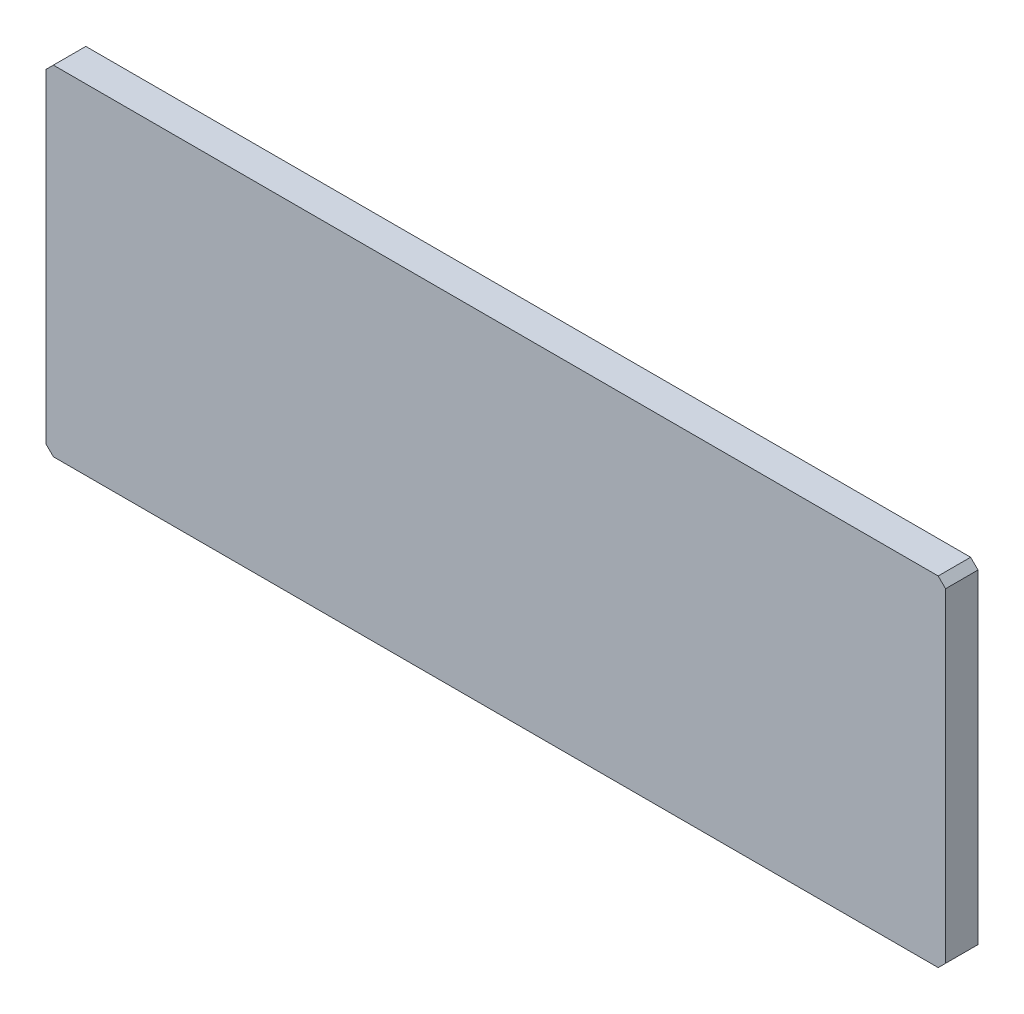
SolidWorks part; units mm, degrees
ref_plane "Front Plane" through (0, 0, 0) normal (0, 0, 1) x (1, 0, 0)
ref_plane "Top Plane" through (0, 0, 0) normal (0, 1, 0) x (1, 0, 0)
ref_plane "Right Plane" through (0, 0, 0) normal (1, 0, 0) x (0, 0, -1)
sketch "Sketch1" plane through (0, 0, 0) normal (0, 0, 1) x (1, 0, 0)
  line L0 (-46.6185, 212.0282) -> (-46.6185, -17.9718)
  line L1 (-46.6185, 212.0282) -> (563.3815, 212.0282)
  line L2 (563.3815, 212.0282) -> (563.3815, -17.9718)
  line L3 (563.3815, -17.9718) -> (-46.6185, -17.9718)
extrude "Boss-Extrude1" add sketch "Sketch1" along normal blind 22
chamfer "Chamfer1" distance 5 angle 45 4 edges at (563.3815, -17.9718, 11) (563.3815, 212.0282, 11) (-46.6185, -17.9718, 11) (-46.6185, 212.0282, 11)
